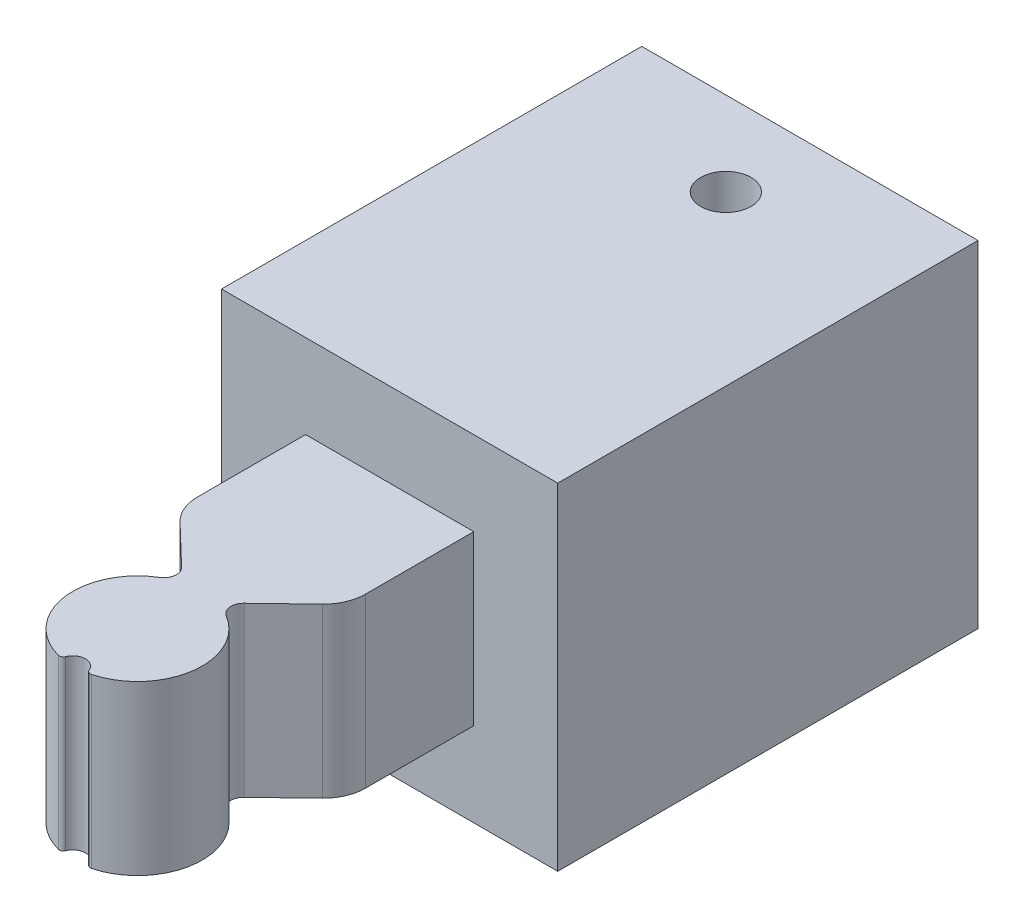
SolidWorks part; units mm, degrees
ref_plane "Front Plane" through (0, 0, 0) normal (0, 0, 1) x (1, 0, 0)
ref_plane "Top Plane" through (0, 0, 0) normal (0, 1, 0) x (1, 0, 0)
ref_plane "Right Plane" through (0, 0, 0) normal (1, 0, 0) x (0, 0, -1)
sketch "Sketch1" plane through (0, 0, 0) normal (0, 1, 0) x (1, 0, 0)
  line L0 (8.4632, -41.4758) -> (3.711, -46.0391)
  line L1 (-20, -25) -> (-10, -25)
  line L2 (-20, -25) -> (-20, 25)
  line L3 (-20, 25) -> (20, 25)
  line L4 (20, -25) -> (20, 25)
  line L5 (-20, -25) -> (20, 25) construction
  line L6 (-20, 25) -> (20, -25) construction
  line L8 (-10, -25) -> (-10, -37.8693)
  line L10 (10, -25) -> (10, -37.8693)
  line L11 (-8.4632, -41.4758) -> (-3.711, -46.0391)
  line L12 (10, -25) -> (20, -25)
  arc A0 (-3.9755, -48.4057) -> (-1.9856, -62.4396) centre (0, -55) ccw
  arc A1 (-3.9755, -48.4057) -> (-3.711, -46.0391) centre (-4.75, -47.1211) ccw
  arc A2 (3.711, -46.0391) -> (3.9755, -48.4057) centre (4.75, -47.1211) ccw
  arc A3 (1.3925, -62.1424) -> (-1.3925, -62.1424) centre (0, -62.7) ccw
  arc A4 (1.9856, -62.4396) -> (3.9755, -48.4057) centre (0, -55) ccw
  arc A5 (1.3925, -62.1424) -> (1.9856, -62.4396) centre (1.8567, -61.9565) ccw
  arc A6 (-1.3925, -62.1424) -> (-1.9856, -62.4396) centre (-1.8567, -61.9565) cw
  arc A7 (8.4632, -41.4758) -> (10, -37.8693) centre (5, -37.8693) ccw
  arc A8 (-10, -37.8693) -> (-8.4632, -41.4758) centre (-5, -37.8693) ccw
  point P0 (0, 0)
  point P22 (1.4929, -62.5539)
  point P27 (10, -40)
  point P30 (-10, -40)
  dimension "D3" = 15.4
  dimension "D8" = 3
  dimension "D9" = 3
  dimension "D11" = 3
  dimension "D12" = 0.5
  dimension "D13" = 5
  dimension "D1" = 50
  dimension "D2" = 40
  dimension "D4" = 80
  dimension "D5" = 15
  dimension "D6" = 20
  dimension "D7" = 10
  dimension "D10" = 9.5
extrude "Boss-Extrude1" add sketch "Sketch1" along normal blind 20
sketch "Sketch2" plane through (0, 20, 0) normal (0, 1, 0) x (1, 0, 0)
  line L1 (-20, 25) -> (20, 25)
  line L2 (-20, 25) -> (-20, -25)
  line L3 (-20, -25) -> (20, -25)
  line L4 (20, 25) -> (20, -25)
extrude "Boss-Extrude2" add sketch "Sketch2" along normal blind 10
sketch "Sketch3" plane through (0, 0, 0) normal (0, -1, 0) x (1, 0, 0)
  line L1 (20, -25) -> (-20, -25)
  line L2 (20, -25) -> (20, 25)
  line L3 (20, 25) -> (-20, 25)
  line L4 (-20, -25) -> (-20, 25)
extrude "Boss-Extrude3" add sketch "Sketch3" along normal blind 10
sketch "Sketch4" plane through (0, -10, 0) normal (0, -1, 0) x (1, 0, 0)
  line L0 (-20, -25) -> (20, -25) construction
  circle A0 centre (0, -15) radius 3
  dimension "D1" = 6
  dimension "D2" = 10
extrude "Cut-Extrude1" cut sketch "Sketch4" against normal blind 59
